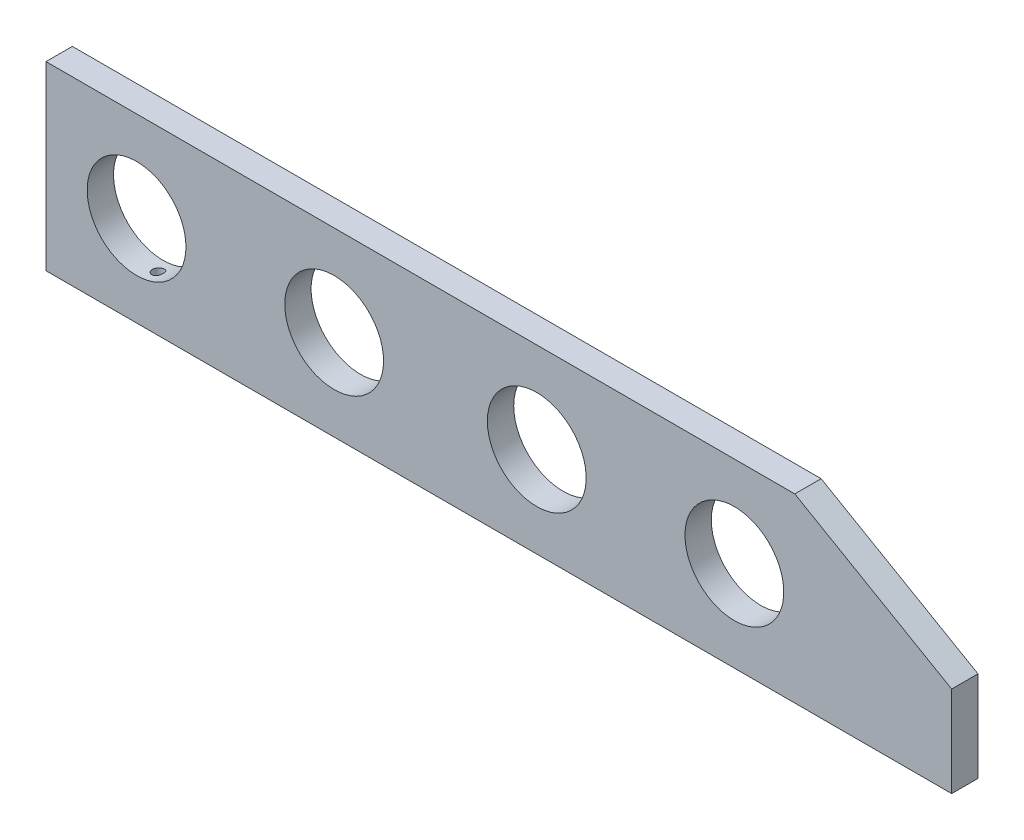
from build123d import *

# Parameters (mm, degrees)
SKETCH_1_W               = 550
SKETCH_1_H               = 110
EXTRUDE_1_DEPTH          = 8
CUT_EXTRUDE_4_DEPTH      = 281.902118184
CUT_EXTRUDE_4_DEPTH_BACK = 281.902118184
HOLE1_D                  = 6.75
HOLE1_DEPTH              = 26
HOLE1_TIP                = 2.027904589
HOLE11_D                 = 6.75
HOLE11_DEPTH             = 28
HOLE11_TIP               = 2.027904589
SKETCH_10_R              = 30
CUT_EXTRUDE_5_DEPTH      = 281.902118184


with BuildPart() as part:
    # 草图1 → 凸台-拉伸1 (new, symmetric)
    with BuildSketch(Plane.XY):
        Rectangle(SKETCH_1_W, SKETCH_1_H)
    extrude(amount=EXTRUDE_1_DEPTH, both=True)

    # 草图9 → 切除-拉伸4 (cut, two sides: drawn at the far end of the back side and taken through both)
    with BuildSketch(Plane.XY.offset(8).offset(-CUT_EXTRUDE_4_DEPTH_BACK)):
        Polygon((-786.302283658, 612.743159162), (179.737205584, 55), (275, 0), (1241.039489242, -557.743159162), (2356.525807565, 1374.335819322), (329.184034665, 2544.822137646), align=None)
    extrude(amount=CUT_EXTRUDE_4_DEPTH + CUT_EXTRUDE_4_DEPTH_BACK, mode=Mode.SUBTRACT)

    # Hole1
    with Locations(Plane(origin=(-134.213455343, -55, 9.167765698), x_dir=(1, 0, 0), z_dir=(0, -1, 0))):
        with Locations((-80.786544657, -9.167765698), (119.213455343, -9.167765698), (369.213455343, -9.167765698)):
            Hole(HOLE1_D / 2, depth=HOLE1_DEPTH)
            with Locations((0, 0, -(HOLE1_DEPTH + HOLE1_TIP / 2))):  # 118° drill point
                Cone(0, HOLE1_D / 2, HOLE1_TIP, mode=Mode.SUBTRACT)

    # Hole11
    with Locations(Plane(origin=(-275, -17.832234302, -14.213455343), x_dir=(0, 0, 1), z_dir=(-1, 0, 0))):
        with Locations((14.213455343, -9.167765698), (14.213455343, 62.832234302)):
            Hole(HOLE11_D / 2, depth=HOLE11_DEPTH)
            with Locations((0, 0, -(HOLE11_DEPTH + HOLE11_TIP / 2))):  # 118° drill point
                Cone(0, HOLE11_D / 2, HOLE11_TIP, mode=Mode.SUBTRACT)

    # 草图10 → 切除-拉伸5 (cut, through all)
    with BuildSketch(Plane.XY.offset(8)):
        with Locations((-220, 0)):
            Circle(SKETCH_10_R)
        with Locations((-100, 0)):
            Circle(SKETCH_10_R)
        with Locations(Location((23.038475773, 0, 0), (0, 0, 180))):
            Circle(SKETCH_10_R)
        with Locations(Location((143.038475773, 0, 0), (0, 0, 180))):
            Circle(SKETCH_10_R)
    extrude(amount=-CUT_EXTRUDE_5_DEPTH, mode=Mode.SUBTRACT)


solid = part.part
